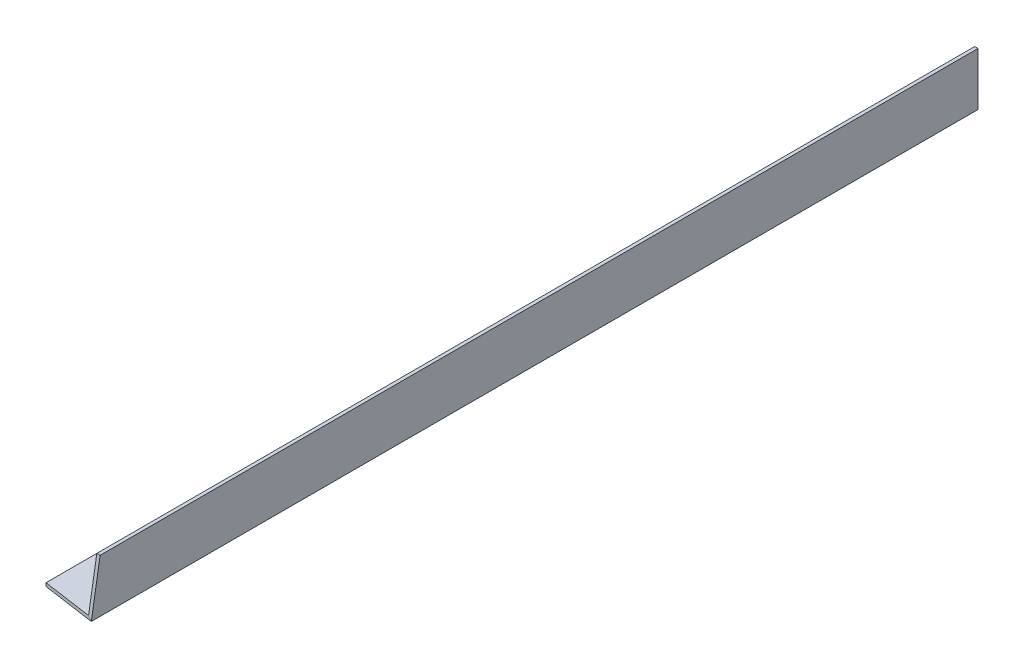
from build123d import *

# Parameters (mm, degrees)
BOSS_EXTRUDE1_DEPTH = 1063.8155
CUT_EXTRUDE1_DEPTH  = 150
SKETCH3_R           = 7.14375
CUT_EXTRUDE2_DEPTH  = 150


with BuildPart() as part:
    # Sketch1 → Boss-Extrude1 (new, symmetric)
    with BuildSketch(Plane.XY):
        Polygon((-127, 0), (0, 0), (0, 127), (-7.9375, 127), (-7.9375, 7.9375), (-127, 7.9375), align=None)
    extrude(amount=BOSS_EXTRUDE1_DEPTH, both=True)

    # Sketch2 → Cut-Extrude1 (cut)
    with BuildSketch(Plane(origin=(0, 0, 0), x_dir=(0, 0, -1), z_dir=(1, 0, 0))):
        Polygon((-1063.8155, 0), (-1063.8155, 127), (-1042.676904036, 127), align=None)
    extrude(amount=-CUT_EXTRUDE1_DEPTH, mode=Mode.SUBTRACT)

    # Sketch3 → Cut-Extrude2 (cut)
    with BuildSketch(Plane.XZ):
        with Locations(Location((-88.9, 879.2845, 0), (0, 0, 270))):
            Circle(SKETCH3_R)
        Polygon((0, 1063.8155), (-127, 1063.8155), (-127, 1045.559770079), align=None)
        with BuildLine():
            Line((-56.35625, -880.45925), (-56.35625, -916.97175))
            ThreePointArc((-56.35625, -916.97175), (-63.5, -924.1155), (-70.64375, -916.97175))
            Line((-70.64375, -916.97175), (-70.64375, -880.45925))
            ThreePointArc((-70.64375, -880.45925), (-63.5, -873.3155), (-56.35625, -880.45925))
        make_face()
    extrude(amount=-CUT_EXTRUDE2_DEPTH, mode=Mode.SUBTRACT)


solid = part.part
